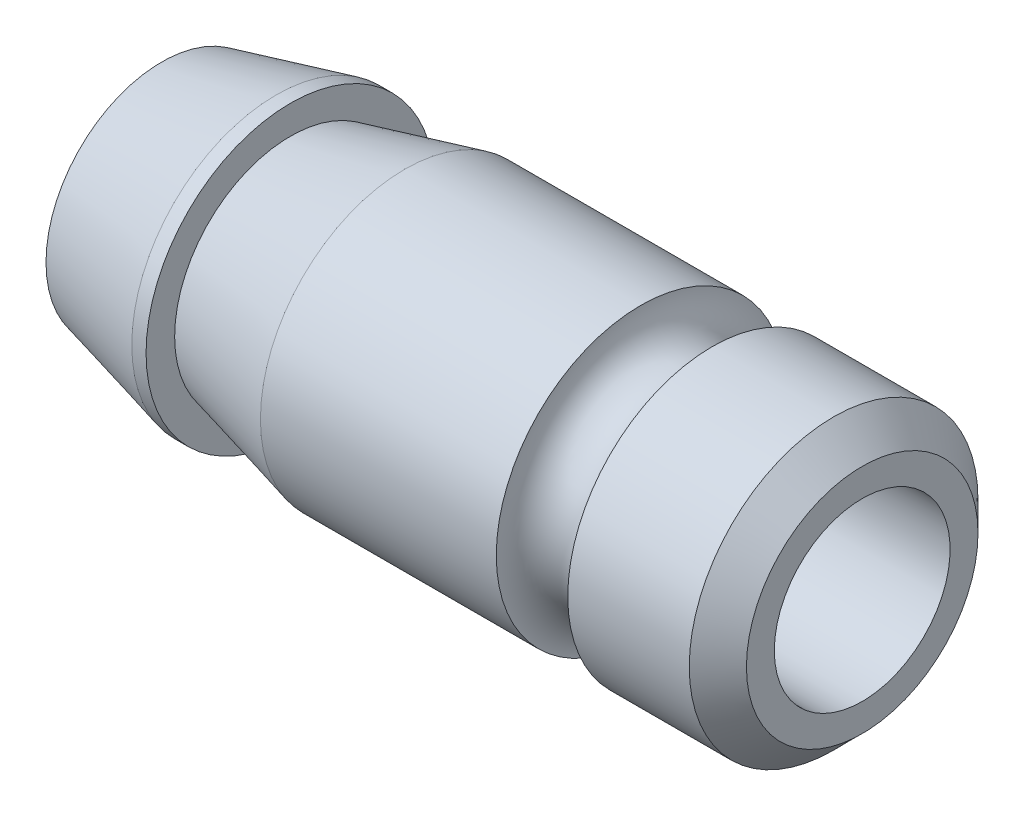
from build123d import *

# Parameters (mm, degrees)
SKETCH2_R          = 6.15
CUT_EXTRUDE1_DEPTH = 99


with BuildPart() as part:
    # Sketch1 → Revolve1 (revolve)
    with BuildSketch(Plane.XY, mode=Mode.PRIVATE) as revolve1_sk:
        with BuildLine():
            Line((17.000000001, 10.1), (9.000000001, 8.100000002))
            Line((9.000000001, 8.100000002), (9.000000001, 10.1))
            Line((9.000000001, 10.1), (8.000000001, 10.1))
            Line((8.000000001, 10.1), (0, 8.100000002))
            Line((0, 8.100000002), (0, 0))
            Line((0, 0), (49, 0))
            Line((49, 0), (49, 8.099999999))
            Line((49, 8.099999999), (46.999999999, 10.1))
            Line((46.999999999, 10.1), (38.500000001, 10.1))
            ThreePointArc((38.500000001, 10.1), (36.000000001, 7.6), (33.500000001, 10.1))
            Line((33.500000001, 10.1), (17.000000001, 10.1))
        make_face()
    revolve(revolve1_sk.sketch.rotate(Axis((0, 0, 0), (1, 0, 0)), 90), axis=Axis((0, 0, 0), (1, 0, 0)))

    # Sketch2 → Cut-Extrude1 (cut)
    with BuildSketch(Plane.ZY):
        Circle(SKETCH2_R)
    extrude(amount=-CUT_EXTRUDE1_DEPTH, mode=Mode.SUBTRACT)


solid = part.part
